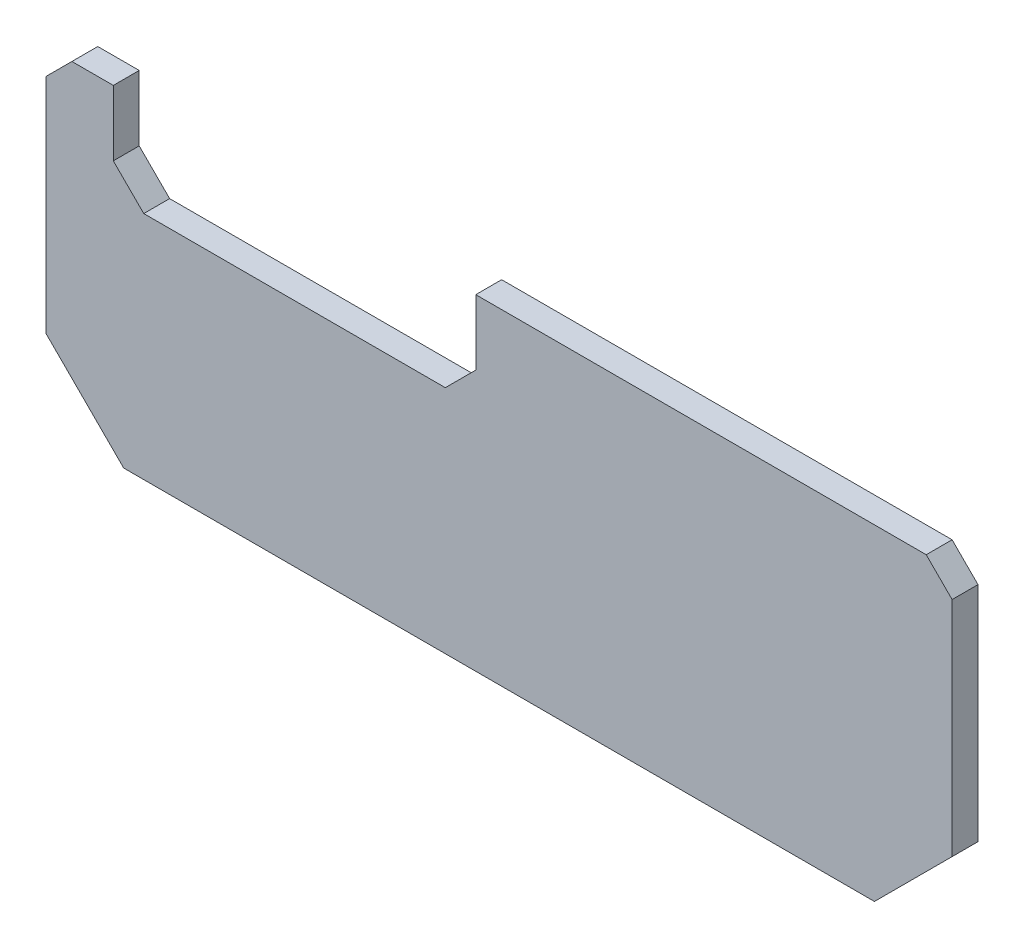
SolidWorks part; units mm, degrees
ref_plane "Front Plane" through (0, 0, 0) normal (0, 0, 1) x (1, 0, 0)
ref_plane "Top Plane" through (0, 0, 0) normal (0, 1, 0) x (1, 0, 0)
ref_plane "Right Plane" through (0, 0, 0) normal (1, 0, 0) x (0, 0, -1)
sketch "Sketch1" plane through (0, 0, 0) normal (0, 0, 1) x (1, 0, 0)
  line L0 (-87.5, 35.8431) -> (-87.5, 42.864) construction
  line L5 (-87.5, 56) -> (87.5, 56)
  line L6 (-87.5, 56) -> (-87.5, -7)
  line L7 (-87.5, -7) -> (87.5, -7)
  line L8 (87.5, 56) -> (87.5, -7)
  line L9 (-74.364, 56) -> (74.364, 56) construction
  line L10 (87.5, 42.864) -> (87.5, 35.8431) construction
  line L11 (-77, 0) -> (-51.8834, 0) construction
  dimension "D1" = 7
extrude "Boss-Extrude1" add sketch "Sketch1" along normal blind 5
sketch "Sketch2" plane through (0, 0, 5) normal (0, 0, 1) x (1, 0, 0)
  line L15 (-74.5, 56) -> (-4.5, 56)
  line L20 (-4.5, 43.3787) -> (-4.5, 56)
  line L21 (-10.3787, 37.5) -> (-4.5, 43.3787)
  line L22 (-68.6213, 37.5) -> (-10.3787, 37.5)
  line L23 (-74.5, 43.3787) -> (-68.6213, 37.5)
  line L24 (-74.5, 56) -> (-74.5, 43.3787)
  line L25 (-4.5, 43.3787) -> (-4.5, 56)
  line L26 (-10.3787, 37.5) -> (-4.5, 43.3787)
  line L27 (-68.6213, 37.5) -> (-10.3787, 37.5)
  line L28 (-74.5, 43.3787) -> (-68.6213, 37.5)
  line L29 (-74.5, 56) -> (-74.5, 43.3787)
  dimension "D1" = 1.5
extrude "Cut-Extrude1" cut sketch "Sketch2" against normal up to surface (5 mm away) up to face at (0, 24.5, 0)
chamfer "Chamfer1" distance 15 angle 45 2 edges at (-87.5, -7, 2.5) (87.5, -7, 2.5)
chamfer "Chamfer2" distance 5 angle 45 2 edges at (87.5, 56, 2.5) (-87.5, 56, 2.5)
sketch "Sketch3" plane through (0, -7, 0) normal (0, -1, 0) x (1, 0, 0)
  line L0 (-38.5, 0) -> (-38.5, -3) construction
  line L1 (-72.5, 0) -> (72.5, 0) construction
  line L2 (-23.5, -3) -> (-53.5, -3)
  line L3 (-53.5, -3) -> (-51.7679, 0)
  line L4 (-51.7679, 0) -> (-25.2321, 0)
  line L5 (-23.5, -3) -> (-25.2321, 0)
  line L6 (0, 0) -> (0, 25.999) construction
  line L7 (-53.5, -3) -> (-51.7679, 0)
  line L8 (-23.5, -3) -> (-25.2321, 0)
  line L9 (-53.5, -3) -> (-51.7679, 0)
  line L10 (-23.5, -3) -> (-25.2321, 0)
  line L11 (-53.5, -3) -> (-51.7679, 0)
  line L12 (-23.5, -3) -> (-25.2321, 0)
  line L13 (23.5, -3) -> (25.2321, 0)
  line L14 (23.5, -3) -> (53.5, -3)
  line L15 (51.7679, 0) -> (25.2321, 0)
  line L16 (53.5, -3) -> (51.7679, 0)
  line M3 (-72.5, 0) -> (72.5, 0)
  dimension "D1" = 3
  dimension "D2" = 60
  dimension "D3" = 30
  dimension "D4" = 38.5
extrude "Boss-Extrude2" add sketch "Sketch3" against normal blind 25 from surface at -7 contours L14 L16 L13 M3 | L2 L5 L3 M3
sketch "Sketch4" plane through (0, 25, 0) normal (0, 1, 0) x (1, 0, 0)
  line L0 (-10.3787, 0) -> (-68.6213, 0) construction
  line L1 (-73.5, 0) -> (-5.5, 0)
  line L2 (-73.5, 0) -> (-73.5, 5)
  line L3 (-73.5, 5) -> (-5.5, 5)
  line L4 (-5.5, 0) -> (-5.5, 5)
  line L7 (-5, 0) -> (-5, 245) construction
  line L8 (-74, 245) -> (-74, 0) construction
  line L9 (73.5, 0) -> (73.5, 5)
  line L10 (82.5, 0) -> (-4.5, 0) construction
  line L11 (73.5, 5) -> (3.5, 5)
  line L12 (3.5, 5) -> (3.5, 0)
  line L15 (74, 0) -> (74, 217) construction
  line L16 (3.5, 0) -> (73.5, 0)
  line L17 (3, 0) -> (3, 217) construction
  line L18 (55.3, 5) -> (21.7, 5) construction
  line L19 (-5, 5) -> (-74, 5) construction
  dimension "D1" = 0.5
  dimension "D2" = 0.5
  dimension "D3" = 0.5
  dimension "D4" = 0.5
extrude "Boss-Extrude3" add sketch "Sketch4" against normal blind 2
